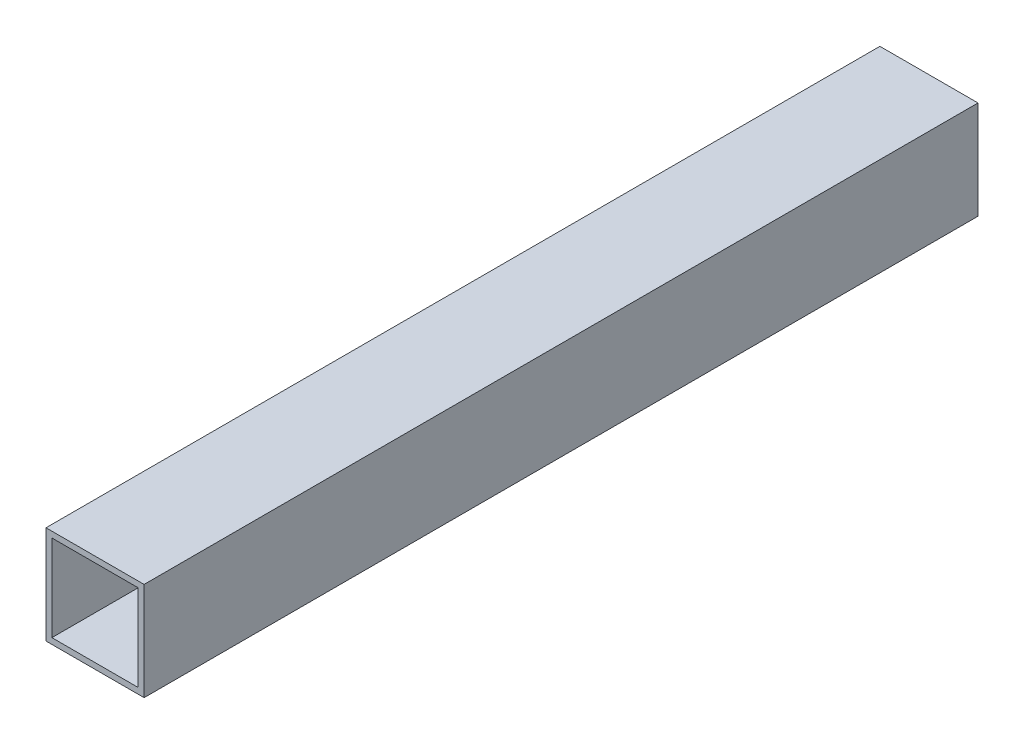
SolidWorks part; units mm, degrees
ref_plane "前视基准面" through (0, 0, 0) normal (0, 0, 1) x (1, 0, 0)
ref_plane "上视基准面" through (0, 0, 0) normal (0, 1, 0) x (1, 0, 0)
ref_plane "右视基准面" through (0, 0, 0) normal (1, 0, 0) x (0, 0, -1)
sketch "草图1" plane through (0, 0, 0) normal (0, 0, 1) x (1, 0, 0)
  line L0 (0, 0) -> (50, 0)
  line L1 (50, 0) -> (50, 50)
  line L2 (50, 50) -> (0, 50)
  line L3 (0, 50) -> (0, 0)
  line L4 (3, 3) -> (47, 3)
  line L5 (47, 3) -> (47, 47)
  line L6 (47, 47) -> (3, 47)
  line L7 (3, 47) -> (3, 3)
  dimension "D1" = 3
extrude "凸台-拉伸1" add sketch "草图1" along normal blind 400
sketch "草图2" plane through (0, 0, 0) normal (0, 0, -1) x (-1, 0, 0)
  line L8 (-47, 47) -> (-47, 3)
  line L9 (-47, 3) -> (-3, 3)
  line L10 (-3, 3) -> (-3, 47)
  line L11 (-3, 47) -> (-47, 47)
  line L12 (0, 0) -> (0, 50)
  line L13 (0, 50) -> (-50, 50)
  line L14 (-50, 50) -> (-50, 0)
  line L15 (-50, 0) -> (0, 0)
  line L16 (0, 0) -> (0, 50)
  line L17 (0, 50) -> (-50, 50)
  line L18 (-50, 50) -> (-50, 0)
  line L19 (-50, 0) -> (0, 0)
  dimension "D1" = 0
extrude "切除-拉伸1" cut sketch "草图2" against normal blind 25
sketch "草图3" plane through (0, 0, 25) normal (0, 0, -1) x (-1, 0, 0)
  line L4 (-47, 47) -> (-47, 3)
  line L5 (-47, 3) -> (-3, 3)
  line L6 (-3, 3) -> (-3, 47)
  line L7 (-3, 47) -> (-47, 47)
  line L8 (-50, 0) -> (0, 0)
  line L9 (0, 0) -> (0, 50)
  line L10 (0, 50) -> (-50, 50)
  line L11 (-50, 50) -> (-50, 0)
  line L12 (-50, 0) -> (0, 0)
  line L13 (0, 0) -> (0, 50)
  line L14 (0, 50) -> (-50, 50)
  line L15 (-50, 50) -> (-50, 0)
  dimension "D1" = 0
extrude "凸台-拉伸2" add sketch "草图3" along normal blind 50
